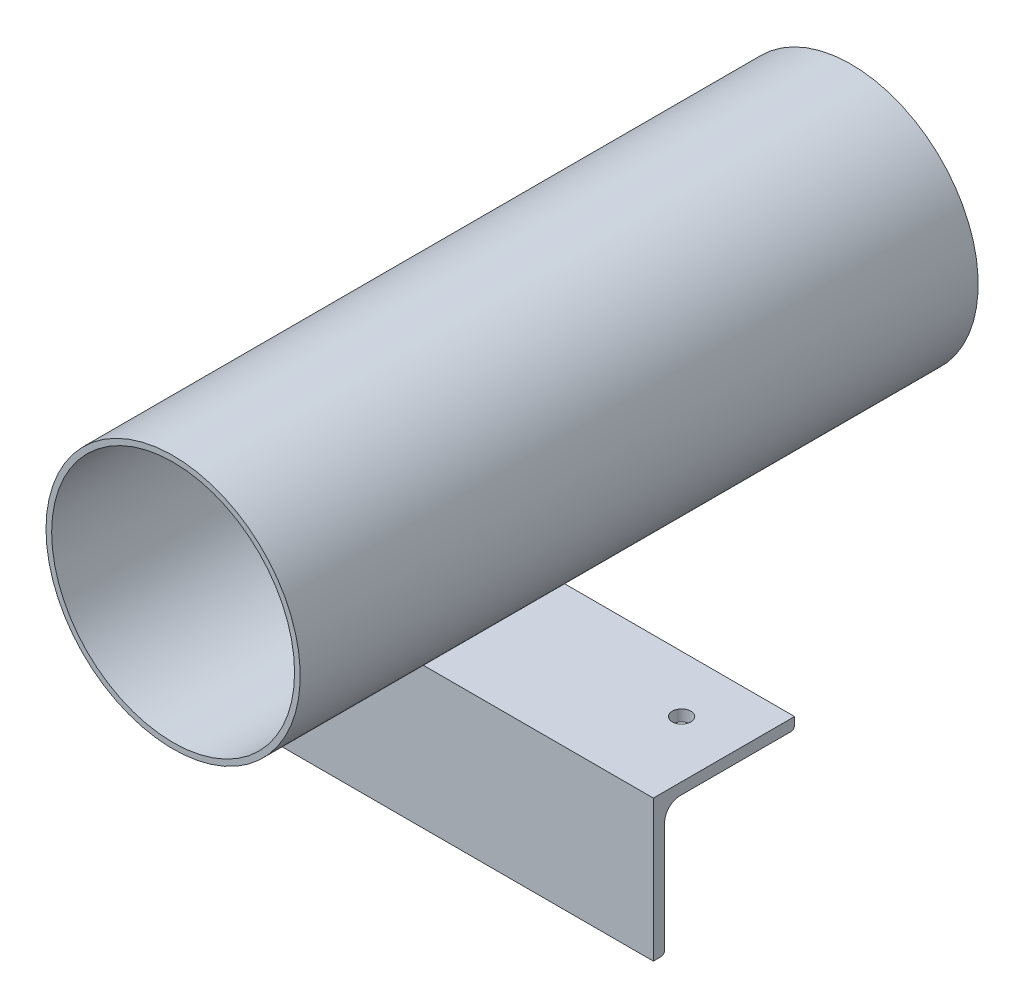
from build123d import *

# Parameters (mm, degrees)
EQUAL_ANGLE_STEEL_5X4_1_DEPTH = 200
BOSS_EXTRUDE1_START           = 120
SKETCH3_R                     = 45
SKETCH3_R_2                   = 43
BOSS_EXTRUDE1_DEPTH           = 240
M6_CLEARANCE_HOLE1_AT_2_COUNT = 2
M6_CLEARANCE_HOLE1_AT_2_PITCH = 160


with BuildPart() as part:
    # Sketch1 → Equal Angle Steel 5X4(1) (new body)
    with BuildSketch(Plane(origin=(0, 0, 0), x_dir=(0, 0, -1), z_dir=(1, 0, 0))):
        with BuildLine():
            Line((50, 0), (0, 0))
            Line((0, 0), (0, -50))
            Line((0, -50), (2.666666667, -50))
            ThreePointArc((2.666666667, -50), (3.609475708, -49.609475708), (4, -48.666666667))
            Line((4, -48.666666667), (4, -9.5))
            ThreePointArc((4, -9.5), (5.610912703, -5.610912703), (9.5, -4))
            Line((9.5, -4), (48.666666667, -4))
            ThreePointArc((48.666666667, -4), (49.609475708, -3.609475708), (50, -2.666666667))
            Line((50, -2.666666667), (50, 0))
        make_face()
    extrude(amount=EQUAL_ANGLE_STEEL_5X4_1_DEPTH)

    # Sketch6 → M6 Clearance Hole1 (revolve, cut)
    with BuildSketch(Plane(origin=(20, 0, -30), x_dir=(0, 0, 1), z_dir=(1, 0, 0))):
        Polygon((0, 0), (0, 21.982840043), (3.3, 20), (3.3, 0), align=None)
    m6_clearance_hole1 = revolve(axis=Axis((20, 6.35, -30), (0, -1, 0)), mode=Mode.SUBTRACT)

    # M6 Clearance Hole1 at 2: M6 Clearance Hole1 ×2
    with Locations(*[(i * M6_CLEARANCE_HOLE1_AT_2_PITCH, 0, 0) for i in range(1, M6_CLEARANCE_HOLE1_AT_2_COUNT)]):
        add(m6_clearance_hole1, mode=Mode.SUBTRACT)


with BuildPart() as body_2:
    # Sketch3 → Boss-Extrude1 (new body)
    with BuildSketch(Plane(origin=(0, 0, -50), x_dir=(-1, 0, 0), z_dir=(0, 0, -1)).offset(BOSS_EXTRUDE1_START)):
        with Locations((-100, 45)):
            Circle(SKETCH3_R)
        with Locations((-100, 45)):
            Circle(SKETCH3_R_2, mode=Mode.SUBTRACT)
    extrude(amount=-BOSS_EXTRUDE1_DEPTH)


solid = Compound([part.part, body_2.part])
